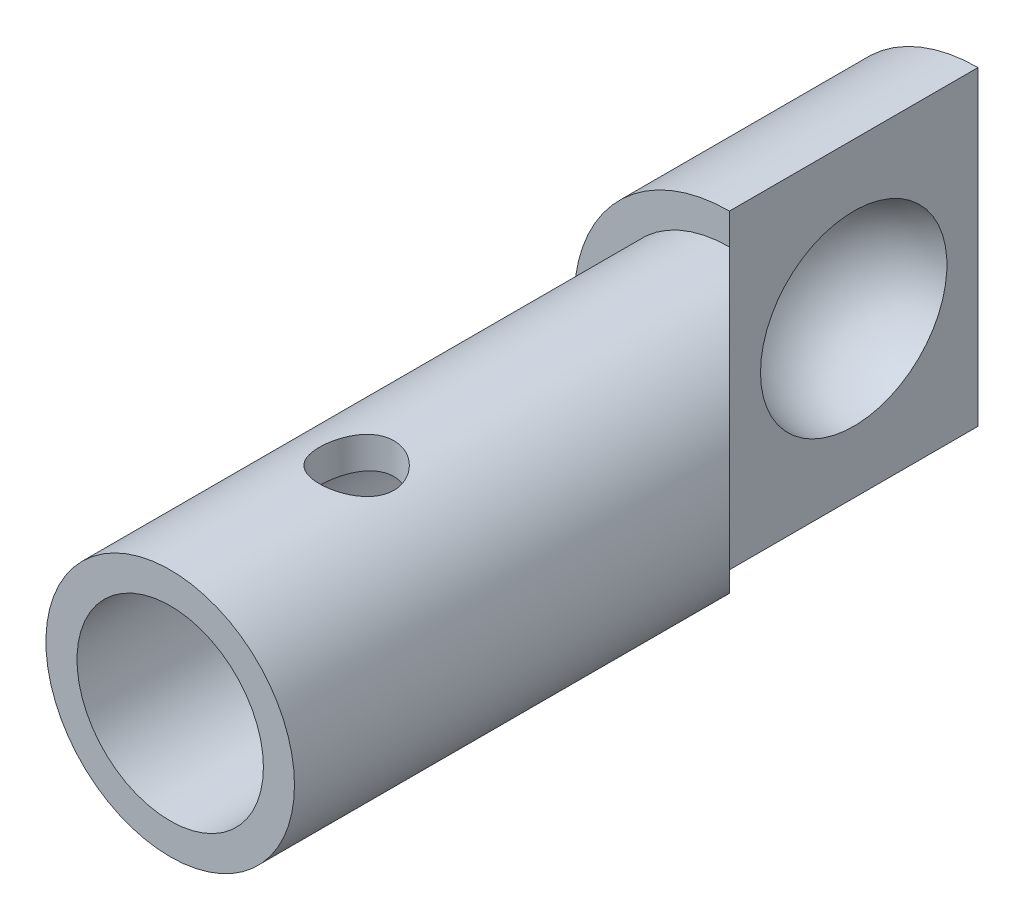
from build123d import *
from build123d.topology import SkipClean

# Parameters (mm, degrees)
SKETCH1_R               = 10
SKETCH1_R_2             = 7.5
BOSS_EXTRUDE1_DEPTH     = 45
CUT_EXTRUDE1_DEPTH      = 48.16990566
CUT_EXTRUDE1_DEPTH_BACK = 48.16990566
SKETCH2_R               = 3
SKETCH3_R               = 12.5
BOSS_EXTRUDE2_DEPTH     = 20
CUT_EXTRUDE2_DEPTH      = 49.347699108
CUT_EXTRUDE2_DEPTH_BACK = 49.347699108


with BuildPart() as part:
    # Sketch1 → Boss-Extrude1 (new body)
    with BuildSketch(Plane.XY):
        with Locations(Location((0, 0, 0), (0, 0, 180))):
            Circle(SKETCH1_R)
        with Locations(Location((0, 0, 0), (0, 0, 180))):
            Circle(SKETCH1_R_2, mode=Mode.SUBTRACT)
    extrude(amount=BOSS_EXTRUDE1_DEPTH)

    # Sketch2 → Cut-Extrude1 (cut, two sides: drawn at the far end of the back side and taken through both)
    with BuildSketch(Plane(origin=(0, 0, 0), x_dir=(1, 0, 0), z_dir=(0, 1, 0)).offset(-CUT_EXTRUDE1_DEPTH_BACK)):
        with Locations(Location((0, -30, 0), (0, 0, 270))):
            Circle(SKETCH2_R)
    extrude(amount=CUT_EXTRUDE1_DEPTH + CUT_EXTRUDE1_DEPTH_BACK, mode=Mode.SUBTRACT)

    # Sketch3 → Boss-Extrude2 (add)
    with BuildSketch(Plane(origin=(0, 0, 0), x_dir=(-1, 0, 0), z_dir=(0, 0, -1))):
        Circle(SKETCH3_R)
    extrude(amount=BOSS_EXTRUDE2_DEPTH)

    # Sketch4 → Cut-Extrude2 (cut, two sides: drawn at the far end of the back side and taken through both)
    with BuildSketch(Plane(origin=(0, 0, 0), x_dir=(1, 0, 0), z_dir=(0, 1, 0)).offset(-CUT_EXTRUDE2_DEPTH_BACK)):
        Polygon((0, 20), (12.5, 20), (12.5, 0), (10, -10), (0, 0), align=None)
    extrude(amount=CUT_EXTRUDE2_DEPTH + CUT_EXTRUDE2_DEPTH_BACK, mode=Mode.SUBTRACT)

    # Sketch5 → Cut-Revolve3 (revolve, cut)
    with SkipClean():  # the faces are left unmerged after this step: merging them gives an invalid solid
        with BuildSketch(Plane(origin=(0, 0, 0), x_dir=(1, 0, 0), z_dir=(0, 1, 0))):
            with BuildLine():
                Line((0, 17.5), (0, 2.5))
                ThreePointArc((0, 2.5), (-7.5, 10), (0, 17.5))
            make_face()
        revolve(axis=Axis((0, 0, 0), (0, 0, -1)), mode=Mode.SUBTRACT)


solid = part.part
